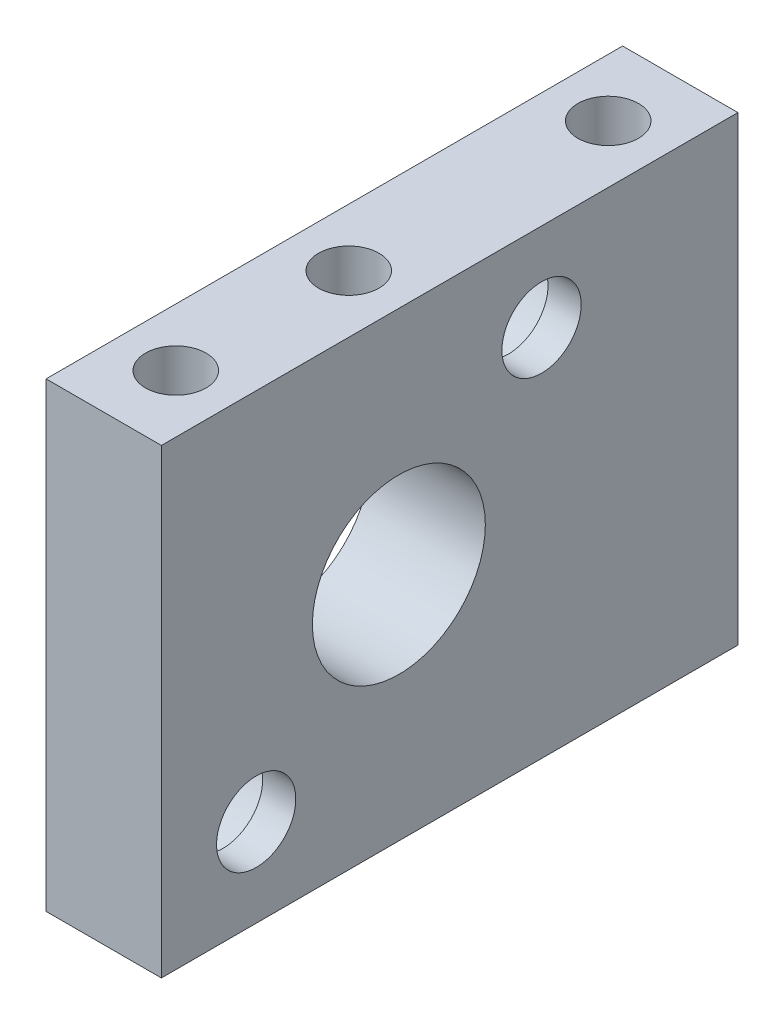
SolidWorks part; units mm, degrees
ref_plane "前视基准面" through (0, 0, 0) normal (0, 0, 1) x (1, 0, 0)
ref_plane "上视基准面" through (0, 0, 0) normal (0, 1, 0) x (1, 0, 0)
ref_plane "右视基准面" through (0, 0, 0) normal (1, 0, 0) x (0, 0, -1)
sketch "草图1" plane through (0, 0, 0) normal (1, 0, 0) x (0, 0, -1)
  line L1 (20, 16) -> (-20, 16)
  line L2 (20, 16) -> (20, -16)
  line L3 (20, -16) -> (-20, -16)
  line L4 (-20, 16) -> (-20, -16)
  line L5 (20, 16) -> (-20, -16) construction
  line L6 (20, -16) -> (-20, 16) construction
  point P0 (0, 0)
  dimension "D1" = 40
  dimension "D2" = 32
extrude "凸台-拉伸1" add sketch "草图1" along normal blind 8
sketch "草图8" plane through (0, 0, 0) normal (-1, 0, 0) x (0, 0, 1)
  line L1 (20, 16) -> (20, -16) construction
  circle A0 centre (3.5237, 0) radius 6
  dimension "D1" = 12
  dimension "D2" = 16.4763
extrude "切除-拉伸2" cut sketch "草图8" against normal through all
hole_wizard "打孔尺寸(%根据)内六角圆柱头螺钉的类型3" positions "草图9" profile "草图10" counterbore size "M5" standard "GB" end condition through all
sketch "草图9" plane through (0, 0, 0) normal (-1, 0, 0) x (0, 0, 1)
  line L0 (-6.3758, 9.8995) -> (13.4231, -9.8995) construction
  line L1 (3.5237, 0) -> (9.181, 1.2618) construction
  line L3 (3.5237, 0) -> (3.5237, 6.4355) construction
  point P0 (-6.3758, 9.8995)
  point P2 (13.4231, -9.8995)
  dimension "D1" = 14
  dimension "D2" = 14
  dimension "D3" = 45
sketch "草图10" plane through (0, 9.8995, -6.3758) normal (0, 1, 0) x (0, 0, 1)
  line L0 (0, 0) -> (0, 8)
  line L1 (0, 8) -> (2.75, 8)
  line L3 (2.75, 8) -> (2.75, 5.7)
  line L4 (2.75, 5.7) -> (5, 5.7)
  line L5 (5, 5.7) -> (5, 0)
  line L7 (5, 0) -> (0, 0)
  line L11 (0, -6.35) -> (0, 107.95) construction
  dimension "通孔孔直径" = 5.5
  dimension "通孔孔深度" = 8
  dimension "柱形沉头孔直径" = 10
  dimension "柱形沉头孔深度" = 5.7
hole_wizard "M5 螺纹孔1" positions "草图11" profile "草图12" tap size "M5" standard "GB"
sketch "草图11" plane through (0, 16, 0) normal (0, 1, 0) x (1, 0, 0)
  line L1 (4, -20) -> (4, -3.8625) construction
  line L2 (8, -20) -> (0, -20) construction
  point P0 (4, -3)
  point P2 (4, -15)
  point P13 (4, 15)
  dimension "D1" = 5
  dimension "D2" = 12
  dimension "D3" = 18
cosmetic thread "孔螺蚊线1" parameters "D1"=10, "D2"=5
cosmetic thread "孔螺蚊线2" parameters "D1"=10, "D2"=5
sketch "草图12" plane through (4, 16, 3) normal (1, 0, 0) x (0, 0, 1)
  line L0 (0, 0) -> (0, 13.6618)
  line L1 (0, 13.6618) -> (2.1, 12.4)
  line L2 (2.1, 12.4) -> (2.1, 0)
  line L5 (2.1, 0) -> (0, 0)
  line L10 (0, 13.6618) -> (-2.1, 12.4) construction
  line L11 (0, -6.35) -> (0, 107.95) construction
  dimension "螺纹孔钻头直径" = 4.2
  dimension "螺纹孔钻头深度" = 12.4
  dimension "导头角度" = 118
cosmetic thread "孔螺蚊线3" parameters "D1"=10, "D2"=5
